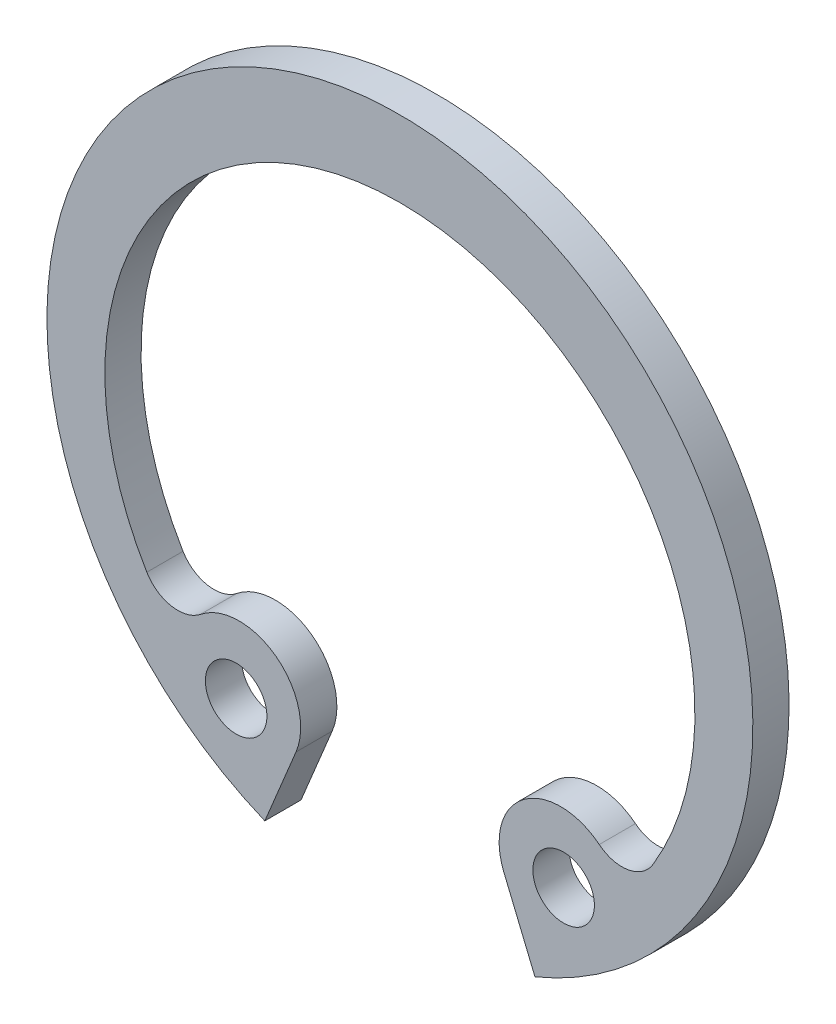
from build123d import *

# Parameters (mm, degrees)
SKETCH_1_R        = 0.85
EXTRUDE_967_DEPTH = 1


with BuildPart() as part:
    # 草图1 → Extrude 967 (new body)
    with BuildSketch(Plane.XY):
        with BuildLine():
            Line((-2.870026243, -6.928856281), (-3.731163466, -9.007825442))
            ThreePointArc((-3.731163466, -9.007825442), (0, 9.75), (3.731163466, -9.007825442))
            Line((3.731163466, -9.007825442), (2.870026243, -6.928856281))
            ThreePointArc((2.870026243, -6.928856281), (3.421390109, -4.91771829), (5.506424922, -4.953884028))
            ThreePointArc((5.506424922, -4.953884028), (6.309138908, -5.1592502), (6.991181868, -4.688779786))
            ThreePointArc((6.991181868, -4.688779786), (0, 7.65), (-6.991181868, -4.688779786))
            ThreePointArc((-6.991181868, -4.688779786), (-6.309138908, -5.1592502), (-5.506424922, -4.953884028))
            ThreePointArc((-5.506424922, -4.953884028), (-3.421390109, -4.91771829), (-2.870026243, -6.928856281))
        make_face()
        with Locations((-4.522967504, -6.47709541)):
            Circle(SKETCH_1_R, mode=Mode.SUBTRACT)
        with Locations(Location((4.522967504, -6.47709541, 0), (0, 0, 180))):
            Circle(SKETCH_1_R, mode=Mode.SUBTRACT)
    extrude(amount=EXTRUDE_967_DEPTH)


solid = part.part
